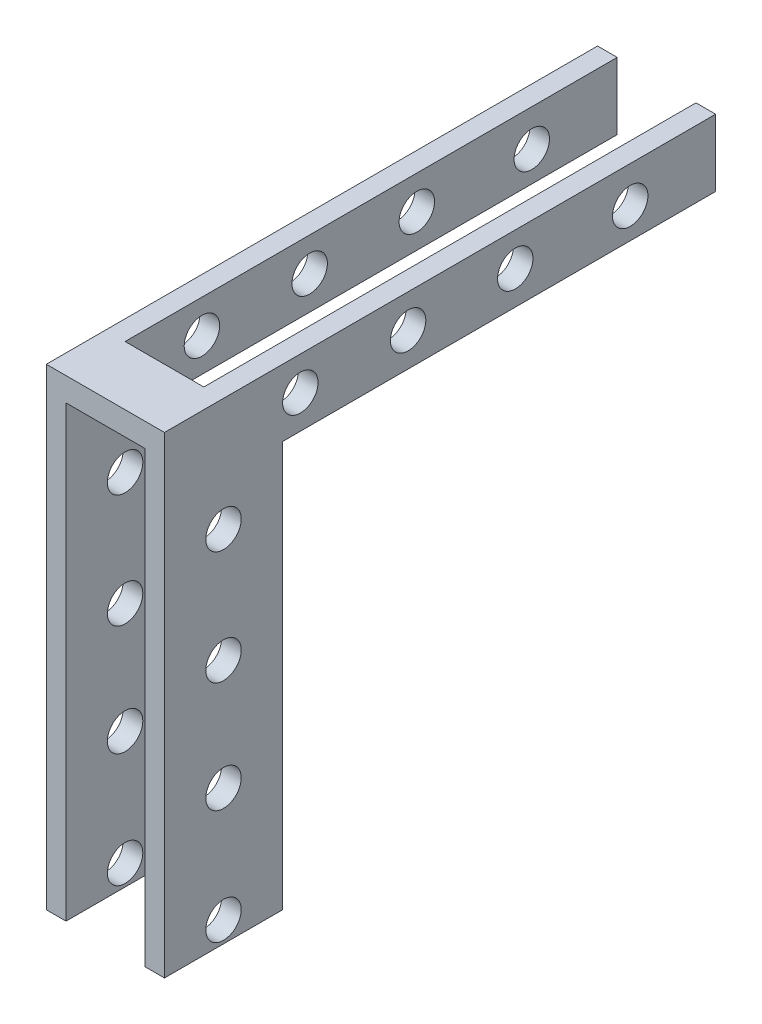
SolidWorks part; units mm, degrees
ref_plane "Front Plane" through (0, 0, 0) normal (0, 0, 1) x (1, 0, 0)
ref_plane "Top Plane" through (0, 0, 0) normal (0, 1, 0) x (1, 0, 0)
ref_plane "Right Plane" through (0, 0, 0) normal (1, 0, 0) x (0, 0, -1)
other "Configuration Table"
sketch "Sketch1" plane through (0, 0, 0) normal (0, 1, 0) x (1, 0, 0)
  line L5 (-100, 150) -> (100, -150) construction
  line L6 (-100, -150) -> (100, 150) construction
  line L7 (100, 150) -> (150, 150)
  line L8 (100, 150) -> (100, -150)
  line L9 (100, -150) -> (150, -150)
  line L10 (150, 150) -> (150, -150)
  line L11 (0, -55) -> (0, 55) construction
  line L12 (-100, -150) -> (-150, -150)
  line L13 (-150, 150) -> (-150, -150)
  line L14 (-100, 150) -> (-150, 150)
  line L15 (-100, 150) -> (-100, -150)
  point P0 (0, 0)
  dimension "D1" = 200
  dimension "D2" = 300
  dimension "D3" = 50
extrude "Boss-Extrude1" add sketch "Sketch1" along normal blind 1200
sketch "Sketch2" plane through (-100, 0, 0) normal (1, 0, 0) x (0, 0, -1)
  line L0 (150, 1200) -> (150, 0) construction
  line L1 (-150, 1200) -> (150, 1200)
  line L2 (-150, 1200) -> (-150, 1140)
  line L3 (-150, 1140) -> (150, 1140)
  line L4 (150, 1200) -> (150, 1140)
  dimension "D1" = 60
extrude "Boss-Extrude2" add sketch "Sketch2" along normal up to next
sketch "Sketch3" plane through (150, 0, 0) normal (1, 0, 0) x (0, 0, -1)
  line L0 (0, 53) -> (0, 0) construction
  line L1 (0, 343) -> (0, 53) construction
  line L2 (0, 624) -> (0, 343) construction
  circle A0 centre (0, 624) radius 45
  circle A1 centre (0, 343) radius 45
  circle A2 centre (0, 53) radius 45
  circle A3 centre (0, 624) radius 45 construction
  dimension "D2" = 290
  dimension "D1" = 53
extrude "Cut-Extrude1" cut sketch "Sketch3" against normal blind 900
sketch "Sketch4" plane through (150, 0, 0) normal (1, 0, 0) x (0, 0, -1)
  circle A0 centre (0, 912.3041) radius 45
sketch "Sketch5" plane through (0, 0, -150) normal (0, 0, -1) x (-1, 0, 0)
  line L0 (-100, 1140) -> (-100, 0) construction
  line L5 (-150, 1200) -> (-100, 1200)
  line L6 (-150, 1200) -> (-150, 1030)
  line L7 (-150, 1030) -> (-100, 1030)
  line L8 (-100, 1200) -> (-100, 1030)
  line L9 (0, 165) -> (0, -165) construction
  line L10 (150, 1030) -> (100, 1030)
  line L11 (100, 1200) -> (100, 1030)
  line L12 (150, 1200) -> (100, 1200)
  line L13 (150, 1200) -> (150, 1030)
  dimension "D1" = 170
extrude "Boss-Extrude3" add sketch "Sketch5" along normal blind 900
sketch "Sketch7" plane through (150, 0, 0) normal (1, 0, 0) x (0, 0, -1)
  line L0 (1050, 1115) -> (-150, 1115) construction
  line L1 (1050, 1200) -> (1050, 1030) construction
  line L2 (-150, 1200) -> (-150, 0) construction
  circle A0 centre (468.8121, 1115) radius 45
  circle A1 centre (741.0135, 1115) radius 45
  circle A2 centre (195.1615, 1115) radius 45
extrude "Cut-Extrude2" cut sketch "Sketch7" against normal blind 900 contours A0 | A1 | A2
sketch "Sketch8" plane through (0, 1200, 0) normal (0, 1, 0) x (1, 0, 0)
  line L0 (100, 1050) -> (100, 150) construction
  line L1 (-100, 150) -> (100, 150)
  line L2 (-100, 150) -> (-100, 0)
  line L3 (-100, 0) -> (100, 0)
  line L4 (100, 150) -> (100, 0)
  dimension "D1" = 150
extrude "Cut-Extrude3" cut sketch "Sketch8" against normal blind 137
sketch "Sketch9" plane through (150, 0, 0) normal (1, 0, 0) x (0, 0, -1)
  circle A0 centre (1032.9517, 1106.8051) radius 45 construction
  circle A1 centre (1032.9517, 1106.8051) radius 45
extrude "Cut-Extrude4" cut sketch "Sketch9" against normal blind 408
sketch "Sketch10" plane through (-150, 0, 0) normal (-1, 0, 0) x (0, 0, 1)
  line L0 (0, 624) -> (0, 912.3041) construction
  circle A0 centre (0, 912.3041) radius 45
  circle A1 centre (0, 624) radius 45 construction
extrude "Cut-Extrude5" cut sketch "Sketch10" against normal blind 997 contours A0
sketch "Sketch11" plane through (0, 0, -1050) normal (0, 0, -1) x (-1, 0, 0)
sketch "Sketch12" plane through (-150, 0, 0) normal (-1, 0, 0) x (0, 0, 1)
  line L0 (-1050, 1200) -> (-1250, 1200)
  line L1 (-1050, 1030) -> (-1250, 1030)
  line L2 (-1250, 1030) -> (-1250, 1200)
  line L4 (-1050, 1200) -> (-1050, 1148.4507)
  line L5 (-1050, 1065.1595) -> (-1050, 1030)
  circle A0 centre (-1032.9517, 1106.8051) radius 45 construction
  arc A1 (-1050, 1148.4507) -> (-1050, 1065.1595) centre (-1032.9517, 1106.8051) ccw
  dimension "D1" = 200
extrude "Boss-Extrude4" add sketch "Sketch12" against normal up to surface (50 mm away) up to face at (-100, 912.3041, 45)
sketch "Sketch13" plane through (150, 0, 0) normal (1, 0, 0) x (0, 0, -1)
  line L5 (1250, 1200) -> (1050, 1200)
  line L6 (1250, 1030) -> (1250, 1200)
  line L7 (1050, 1030) -> (1250, 1030)
  line L8 (1050, 1065.1595) -> (1050, 1030)
  line L9 (1050, 1200) -> (1050, 1148.4507)
  line L10 (1250, 1200) -> (1050, 1200)
  line L11 (1250, 1030) -> (1250, 1200)
  line L12 (1050, 1030) -> (1250, 1030)
  line L13 (1050, 1065.1595) -> (1050, 1030)
  line L14 (1050, 1200) -> (1050, 1148.4507)
  arc A1 (1050, 1065.1595) -> (1050, 1148.4507) centre (1032.9517, 1106.8051) ccw
  arc A2 (1050, 1065.1595) -> (1050, 1148.4507) centre (1032.9517, 1106.8051) ccw
  dimension "D1" = 0
extrude "Boss-Extrude5" add sketch "Sketch13" against normal up to surface (50 mm away) up to face at (100, 912.3041, -45)
